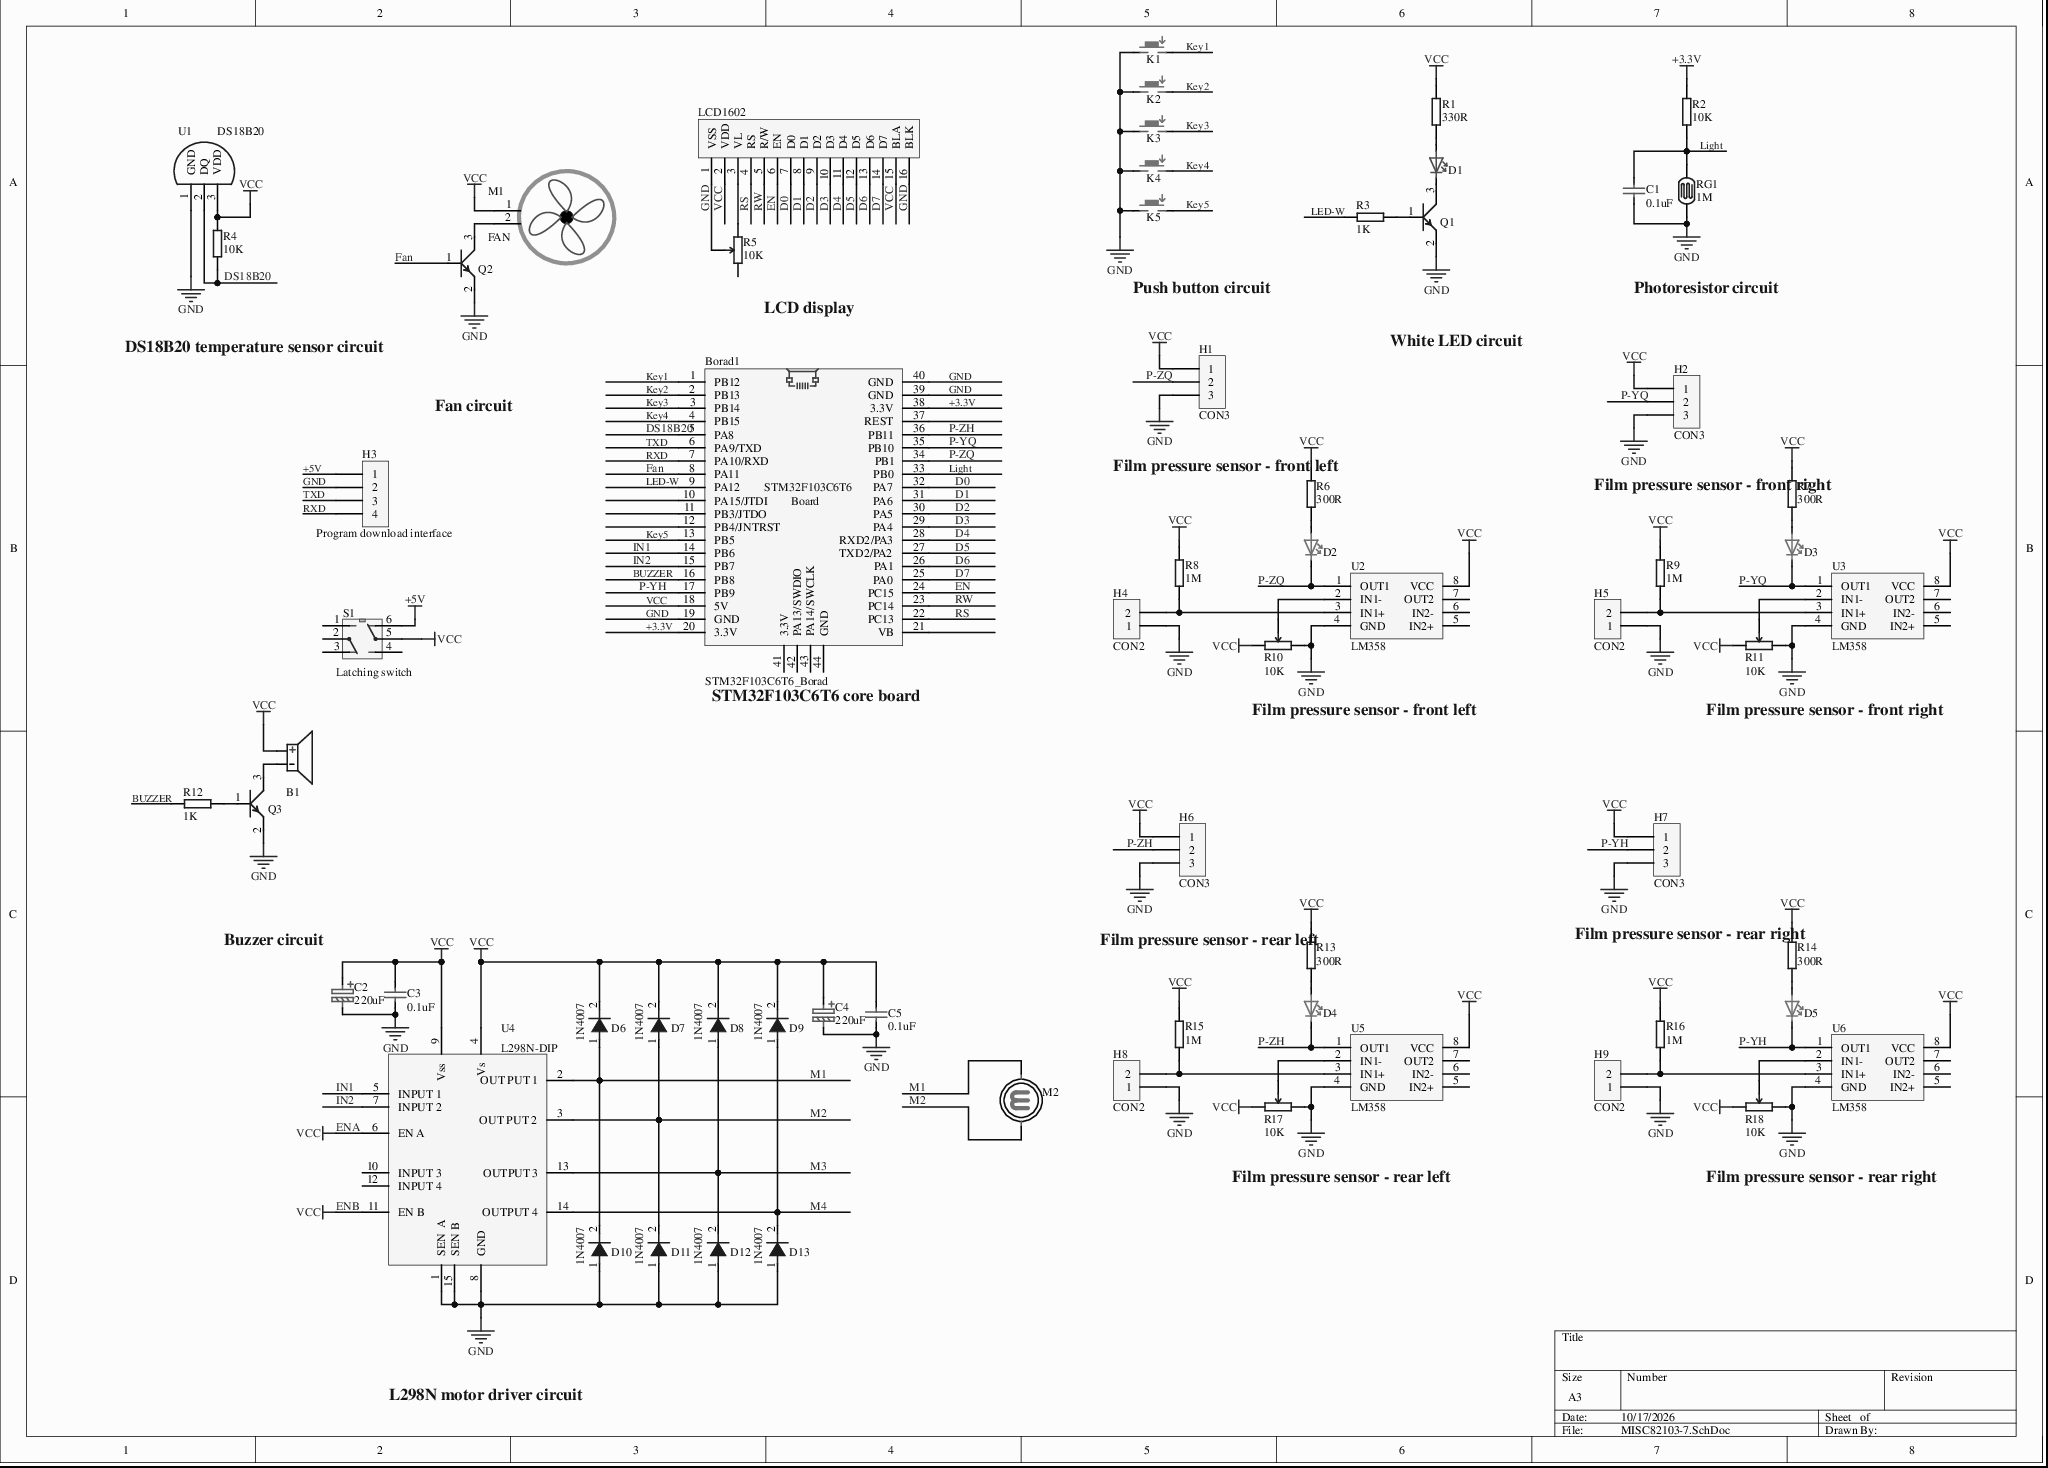
[diagram p0: MISC82103-7.SchDoc]
# Altium project MISC82103-6.PrjPcb
1 sheet, 66 parts. Net scope: global (net labels, ports and power ports of the same name join across sheets).
Board file: MISC82103.PcbDoc

## Sheet MISC82103-7.SchDoc
size A3

### Parts
B1  Buzzer  [BUZZER]  (value not drawn)
Borad1  STM32F103C6T6_Borad  [STM32F103C8T6_买的]
C1  0.1uF  [CAP - 2.54mm]
C2  220uF  [CAPe - 3.5MM]
C3  0.1uF  [CAP - 2.54mm]
C4  220uF  [CAPe - 3.5MM]
C5  0.1uF  [CAP - 2.54mm]
D1  LED  [LED-3MM]  (value not drawn)
D2  LED  [LED-3MM]  (value not drawn)
D3  LED  [LED-3MM]  (value not drawn)
D4  LED  [LED-3MM]  (value not drawn)
D5  LED  [LED-3MM]  (value not drawn)
D6  1N4007  [DIODE - 15.24mm]
D7  1N4007  [DIODE - 15.24mm]
D8  1N4007  [DIODE - 15.24mm]
D9  1N4007  [DIODE - 15.24mm]
D10  1N4007  [DIODE - 15.24mm]
D11  1N4007  [DIODE - 15.24mm]
D12  1N4007  [DIODE - 15.24mm]
D13  1N4007  [DIODE - 15.24mm]
H1  CON3  [CON3]
H2  CON3  [CON3]
H3  Program download interface  [CON4]
H4  CON2  [CON2]
H5  CON2  [CON2]
H6  CON3  [CON3]
H7  CON3  [CON3]
H8  CON2  [CON2]
H9  CON2  [CON2]
K1  Key  [Buttom]  (value not drawn)
K2  Key  [Buttom]  (value not drawn)
K3  Key  [Buttom]  (value not drawn)
K4  Key  [Buttom]  (value not drawn)
K5  Key  [Buttom]  (value not drawn)
LCD1  LCD1602  [LCD1602]
M1  FAN  [CON2]
M2  MOTTOR  [CON2]  (value not drawn)
Q1  NPN  [NPN & PNP]  (value not drawn)
Q2  NPN  [NPN & PNP]  (value not drawn)
Q3  NPN  [NPN & PNP]  (value not drawn)
R1  330R  [Resistor-7.62mm]
R2  10K  [Resistor-7.62mm]
R3  1K  [Resistor-7.62mm]
R4  10K  [Resistor-7.62mm]
R5  10K  [Res_Variable-DIP]
R6  300R  [Resistor-7.62mm]
R7  300R  [Resistor-7.62mm]
R8  1M  [Resistor-7.62mm]
R9  1M  [Resistor-7.62mm]
R10  10K  [Res_Variable-DIP]
R11  10K  [Res_Variable-DIP]
R12  1K  [Resistor-7.62mm]
R13  300R  [Resistor-7.62mm]
R14  300R  [Resistor-7.62mm]
R15  1M  [Resistor-7.62mm]
R16  1M  [Resistor-7.62mm]
R17  10K  [Res_Variable-DIP]
R18  10K  [Res_Variable-DIP]
RG1  1M  [RG]
S1  Latching switch  [Switch]
U1  DS18B20  [DS18B20]
U2  LM358  [DIP8]
U3  LM358  [DIP8]
U4  L298N-DIP  [L298N]
U5  LM358  [DIP8]
U6  LM358  [DIP8]

### Nets
+3.3V: Borad1.20(3.3V) Borad1.38(3.3V) R2.2
+5V: H3.1 S1.6
ENA: B1.1(+) Borad1.18(5V) C2.1 C3.2 C4.1 C5.2 D6.2 D7.2 D8.2 D9.2 H1.1 H2.1 H6.1 H7.1 LCD1.2(VDD) LCD1.15(BLA) M1.1 R1.2 R4.1 R6.2 R7.2 R8.2 R9.2 R10.3 R11.3 R13.2 R14.2 R15.2 R16.2 R17.3 R18.3 S1.5 U1.3(VDD) U2.8(VCC) U3.8(VCC) U4.4(Vs) U4.6(EN_A) U4.9(Vss) U4.11(EN_B) U5.8(VCC) U6.8(VCC)  [also labelled ENB, VCC]
GND: Borad1.19(GND) Borad1.39(GND) Borad1.40(GND) C1.1 C2.2 C3.1 C4.2 C5.1 D10.1 D11.1 D12.1 D13.1 H1.3 H2.3 H3.2 H4.1 H5.1 H6.3 H7.3 H8.1 H9.1 K1.1 K2.1 K3.1 K4.1 K5.1 LCD1.1(VSS) LCD1.16(BLK) Q1.2 Q2.2 Q3.2 R5.2 R10.1 R11.1 R17.1 R18.1 RG1.1 U1.1(GND) U2.4(GND) U3.4(GND) U4.1(SEN__A) U4.8(GND) U4.15(SEN_B) U5.4(GND) U6.4(GND)
BUZZER: Borad1.16(PB8) R12.1
D0: Borad1.32(PA7) LCD1.7(D0)
D1: Borad1.31(PA6) LCD1.8(D1)
D2: Borad1.30(PA5) LCD1.9(D2)
D3: Borad1.29(PA4) LCD1.10(D3)
D4: Borad1.28(RXD2/PA3) LCD1.11(D4)
D5: Borad1.27(TXD2/PA2) LCD1.12(D5)
D6: Borad1.26(PA1) LCD1.13(D6)
D7: Borad1.25(PA0) LCD1.14(D7)
DS18B20: Borad1.5(PA8) R4.2 U1.2(DQ)
EN: Borad1.24(PC15) LCD1.6(EN)
Fan: Borad1.8(PA11) Q2.1
IN1: Borad1.14(PB6) U4.5(INPUT_1)
IN2: Borad1.15(PB7) U4.7(INPUT_2)
Key1: Borad1.1(PB12) K1.2
Key2: Borad1.2(PB13) K2.2
Key3: Borad1.3(PB14) K3.2
Key4: Borad1.4(PB15) K4.2
Key5: Borad1.13(PB5) K5.2
LED-W: Borad1.9(PA12) R3.2
Light: Borad1.33(PB0) C1.2 R2.1 RG1.2
M1: D6.1 D10.2 M2.2 U4.2(OUT_PUT_1)
M2: D7.1 D11.2 M2.1 U4.3(OUT_PUT_2)
M3: D8.1 D12.2 U4.13(OUTPUT_3)
M4: D9.1 D13.2 U4.14(OUTPUT_4)
P-YH: Borad1.17(PB9) D5.1 H7.2 U6.1(OUT1)
P-YQ: Borad1.35(PB10) D3.1 H2.2 U3.1(OUT1)
P-ZH: Borad1.36(PB11) D4.1 H6.2 U5.1(OUT1)
P-ZQ: Borad1.34(PB1) D2.1 H1.2 U2.1(OUT1)
RS: Borad1.22(PC13) LCD1.4(RS)
RW: Borad1.23(PC14) LCD1.5(R/W)
RXD: Borad1.7(PA10/RXD) H3.4
TXD: Borad1.6(PA9/TXD) H3.3
NetB1_2: B1.2(-) Q3.3
NetD1_1: D1.1 Q1.3
NetD1_2: D1.2 R1.1
NetD2_2: D2.2 R6.1
NetD3_2: D3.2 R7.1
NetD4_2: D4.2 R13.1
NetD5_2: D5.2 R14.1
NetH4_2: H4.2 R8.1 U2.3(IN1+)
NetH5_2: H5.2 R9.1 U3.3(IN1+)
NetH8_2: H8.2 R15.1 U5.3(IN1+)
NetH9_2: H9.2 R16.1 U6.3(IN1+)
NetLCD1_3: LCD1.3(VL) R5.1
NetM1_2: M1.2 Q2.3
NetQ1_1: Q1.1 R3.1
NetQ3_1: Q3.1 R12.2
NetR10_2: R10.2 U2.2(IN1-)
NetR11_2: R11.2 U3.2(IN1-)
NetR17_2: R17.2 U5.2(IN1-)
NetR18_2: R18.2 U6.2(IN1-)

Not connected (* = marked no-connect by the designer): Borad1 10(PA15/JTDI) 11(PB3/JTDO) 12(PB4/JNTRST) 21(VB) 37(REST) 41(3.3V) 42(PA13/SWDIO) 43(PA14/SWCLK) 44(GND); R5 3; S1 1 2 3 4; U2 5(IN2+) 6(IN2-) 7(OUT2); U3 5(IN2+) 6(IN2-) 7(OUT2); U4 10(INPUT_3) 12(INPUT_4); U5 5(IN2+) 6(IN2-) 7(OUT2); U6 5(IN2+) 6(IN2-) 7(OUT2)

### Notes on the sheet
- Push button circuit
- Photoresistor circuit
- DS18B20 temperature sensor circuit
- LCD display
- White LED circuit
- Fan circuit
- (near R6) Film pressure sensor - front left
- (near R7) Film pressure sensor - front right
- (near Borad1) STM32F103C6T6 core board
- Film pressure sensor - front left
- Film pressure sensor - front right
- (near C2) Buzzer circuit
- (near R13) Film pressure sensor - rear left
- (near R14) Film pressure sensor - rear right
- Film pressure sensor - rear left
- Film pressure sensor - rear right
- L298N motor driver circuit

### Library data of the parts
Borad1 = STM32F103C6T6_Borad: Core board (purchased online)
C1 C3 C5 = CAP: Non-polar capacitor
C2 C4 = CAP-E: Polar capacitor
D1 = LED-RED
D2-D5 = LED-GREEN
D6-D13 = Diode: Rectifier diode / single-direction diode
H1 H2 H6 H7 = CON3: Pin header / terminal block / connector
H3 = CON4: Pin header / terminal block / connector
H4 H5 H8 H9 = CON2: Pin header / terminal block / connector
K1-K5 = Key: Push button
M1 = FAN: Small fan
M2 = MOTTOR: DC motor
Q1-Q3 = NPN: NPN transistor
R1-R4 R6-R9 R12-R16 = Res: Resistor
R5 R10 R11 R17 R18 = Res_Variable: Adjustable resistor
RG1 = RG: Photoresistor
S1 = Switch: 8*8 power switch / latching switch
U1 = DS18B20: Temperature sensor
U2 U3 U5 U6 = LM358: Dual operational amplifier
U4 = L298N-DIP: Dual H-bridge driver IC